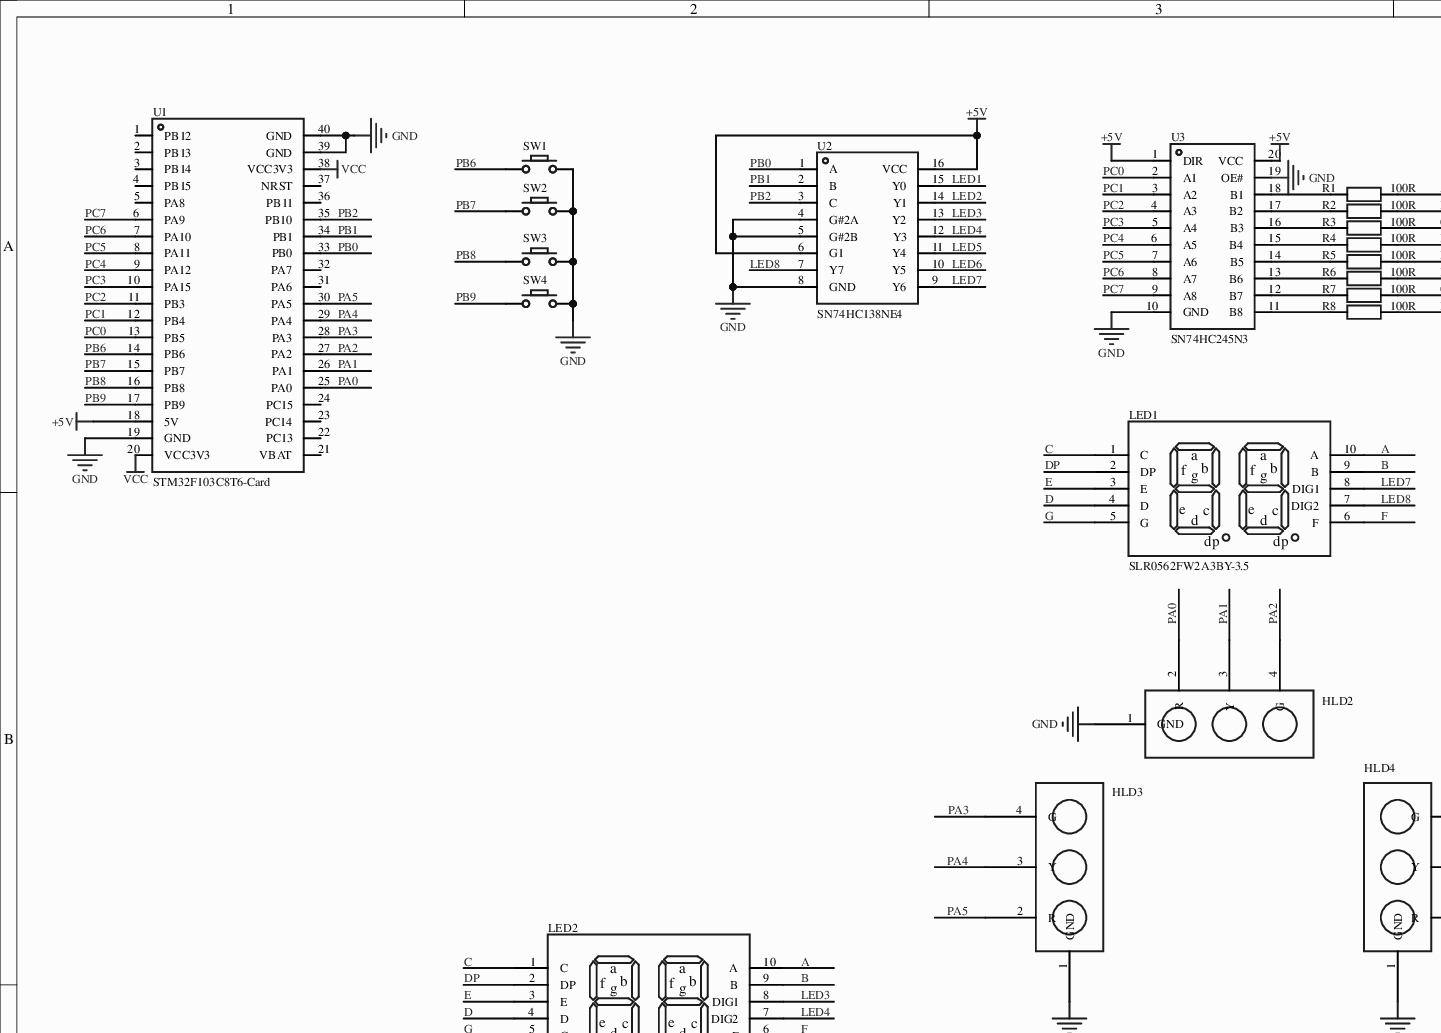
[diagram p0: MISC51569-3.schdoc, top left]
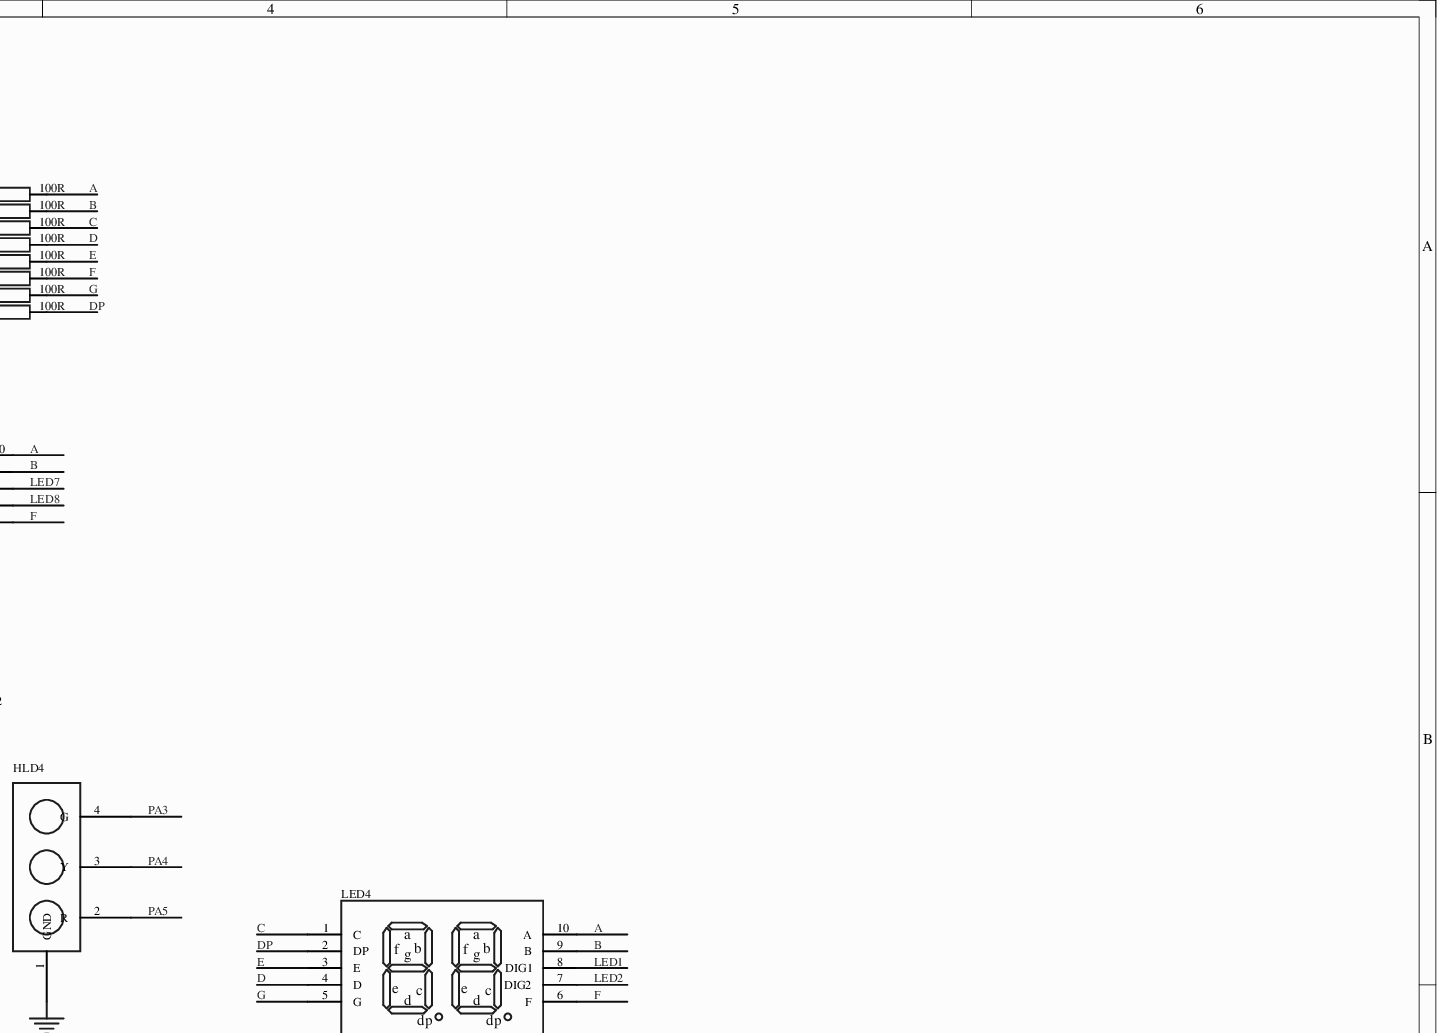
[diagram p1: MISC51569-3.schdoc, top right]
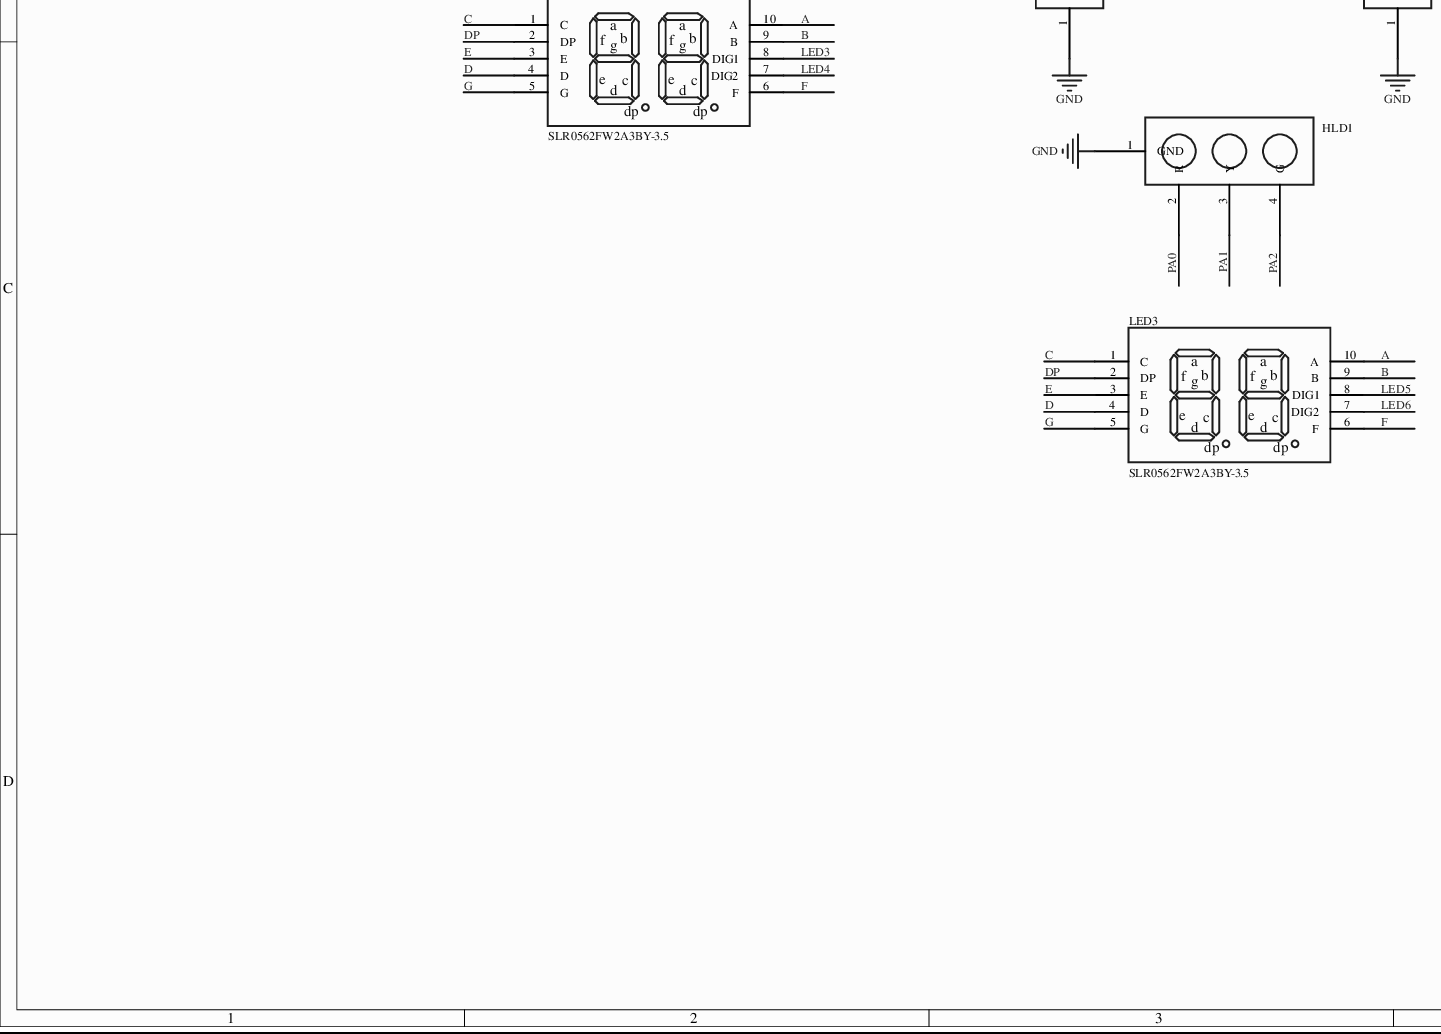
[diagram p2: MISC51569-3.schdoc, bottom left]
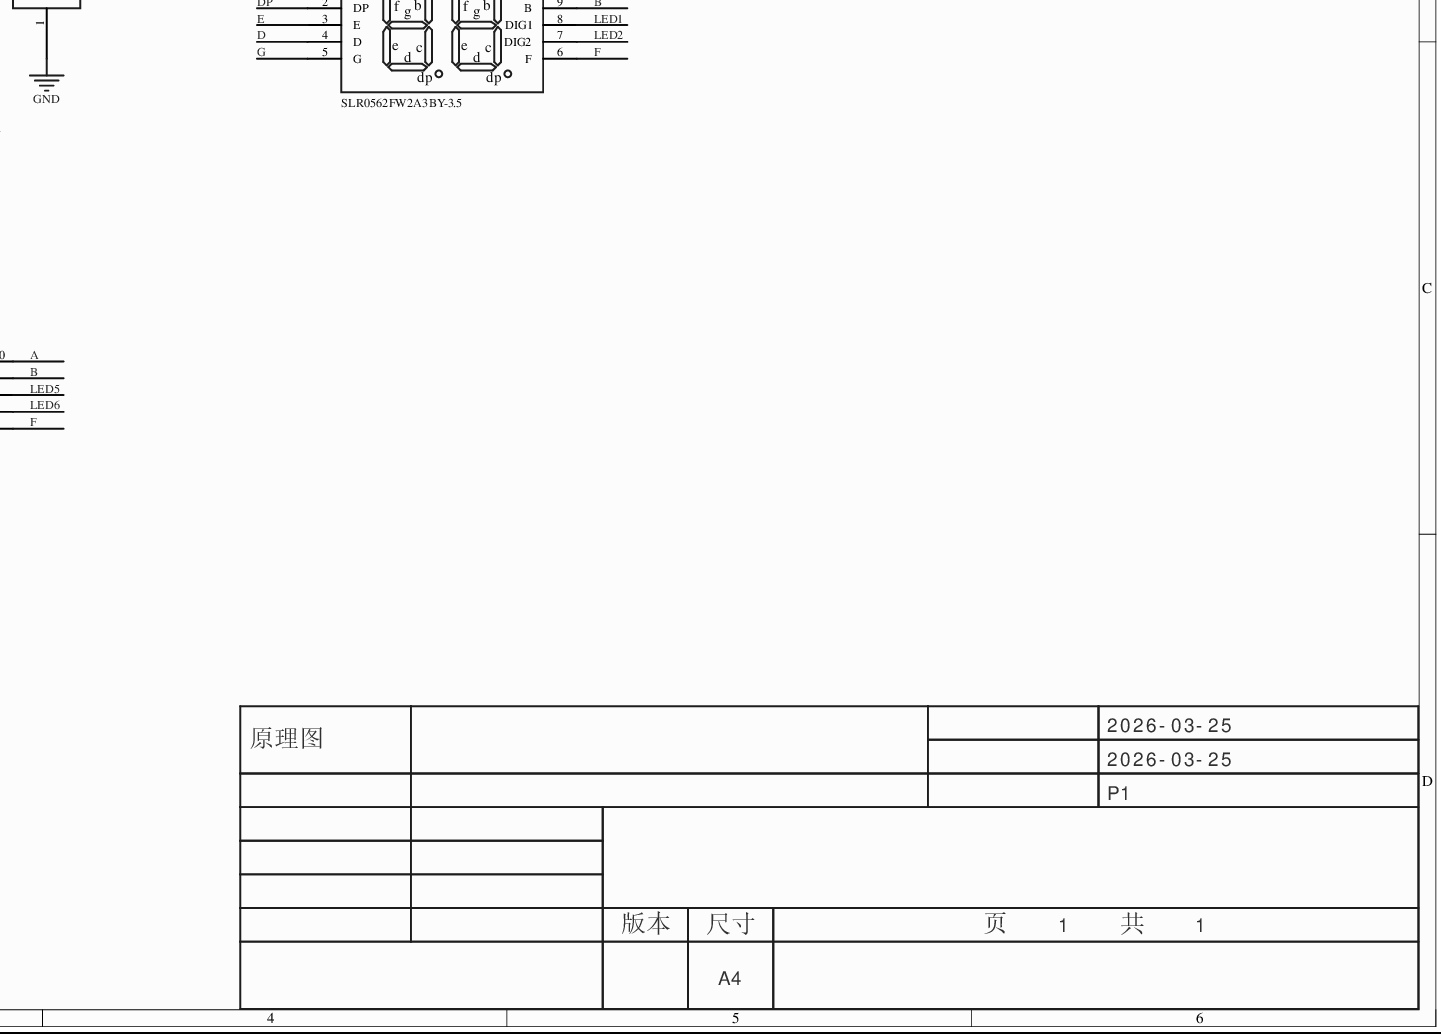
[diagram p3: MISC51569-3.schdoc, bottom right]
# Altium project MISC51569-2.PrjPcb
1 sheet, 23 parts. Net scope: global (net labels, ports and power ports of the same name join across sheets).
Board file: MISC51569.pcbdoc

## Sheet MISC51569-3.schdoc
size 420 x 297 mm; Version: V1.0; @Project Name: MISC51569; @Update Date: 2026-03-25; @Create Date: 2026-03-25; @Board Name: MISC51569; @Create Time: 20:56:41; @Page Count: 1; @Page No: 1; @Schematic Name: MISC51569; @Update Time: 20:56:41; Size: A4

### Parts
HLD1  (no value)  [SIP-04]
HLD2  (no value)  [SIP-04]
HLD3  (no value)  [SIP-04]
HLD4  (no value)  [SIP-04]
LED1  SLR0562FW2A3BY-3.5  [LED-SEG-TH_10P-L25.0-W19.0-P2.54-S15.24-BL]
LED2  SLR0562FW2A3BY-3.5  [LED-SEG-TH_10P-L25.0-W19.0-P2.54-S15.24-BL]
LED3  SLR0562FW2A3BY-3.5  [LED-SEG-TH_10P-L25.0-W19.0-P2.54-S15.24-BL]
LED4  SLR0562FW2A3BY-3.5  [LED-SEG-TH_10P-L25.0-W19.0-P2.54-S15.24-BL]
R1  100R  [Res_1/8W]
R2  100R  [Res_1/8W]
R3  100R  [Res_1/8W]
R4  100R  [Res_1/8W]
R5  100R  [Res_1/8W]
R6  100R  [Res_1/8W]
R7  100R  [Res_1/8W]
R8  100R  [Res_1/8W]
SW1  (no value)  [Key_TH_3.5x6x4.3]
SW2  (no value)  [Key_TH_3.5x6x4.3]
SW3  (no value)  [Key_TH_3.5x6x4.3]
SW4  (no value)  [Key_TH_3.5x6x4.3]
U1  STM32F103C8T6-Card  [CONN-TH_L53.3-W22.9_STM32F103C8T6-CARD]
U2  SN74HC138NE4  [PDIP-16_L19.7-W6.6-P2.54-LS7.6-BL]
U3  SN74HC245N3  [PDIP-20_L25.9-W6.6-P2.54-LS7.9-BL]

### Nets
+5V: U1.18(5V) U2.6(G1) U2.16(VCC) U3.1(DIR) U3.20(VCC)
GND: HLD1.1(GND) HLD2.1(GND) HLD3.1(GND) HLD4.1(GND) SW1.B SW2.B SW3.B SW4.B U1.19(GND) U1.39(GND) U1.40(GND) U2.4(G#2A) U2.5(G#2B) U2.8(GND) U3.10(GND) U3.19(OE#)
VCC: U1.20(VCC3V3) U1.38(VCC3V3)
A: LED1.10(A) LED2.10(A) LED3.10(A) LED4.10(A) R1.2
B: LED1.9(B) LED2.9(B) LED3.9(B) LED4.9(B) R2.2
C: LED1.1(C) LED2.1(C) LED3.1(C) LED4.1(C) R3.2
D: LED1.4(D) LED2.4(D) LED3.4(D) LED4.4(D) R4.2
DP: LED1.2(DP) LED2.2(DP) LED3.2(DP) LED4.2(DP) R8.2
E: LED1.3(E) LED2.3(E) LED3.3(E) LED4.3(E) R5.2
F: LED1.6(F) LED2.6(F) LED3.6(F) LED4.6(F) R6.2
G: LED1.5(G) LED2.5(G) LED3.5(G) LED4.5(G) R7.2
LED1: LED4.8(DIG1) U2.15(Y0)
LED2: LED4.7(DIG2) U2.14(Y1)
LED3: LED2.8(DIG1) U2.13(Y2)
LED4: LED2.7(DIG2) U2.12(Y3)
LED5: LED3.8(DIG1) U2.11(Y4)
LED6: LED3.7(DIG2) U2.10(Y5)
LED7: LED1.8(DIG1) U2.9(Y6)
LED8: LED1.7(DIG2) U2.7(Y7)
PA0: HLD1.2(R) HLD2.2(R) U1.25(PA0)
PA1: HLD1.3(Y) HLD2.3(Y) U1.26(PA1)
PA2: HLD1.4(G) HLD2.4(G) U1.27(PA2)
PA3: HLD3.4(G) HLD4.4(G) U1.28(PA3)
PA4: HLD3.3(Y) HLD4.3(Y) U1.29(PA4)
PA5: HLD3.2(R) HLD4.2(R) U1.30(PA5)
PB0: U1.33(PB0) U2.1(A)
PB1: U1.34(PB1) U2.2(B)
PB2: U1.35(PB10) U2.3(C)
PB6: SW1.A U1.14(PB6)
PB7: SW2.A U1.15(PB7)
PB8: SW3.A U1.16(PB8)
PB9: SW4.A U1.17(PB9)
PC0: U1.13(PB5) U3.2(A1)
PC1: U1.12(PB4) U3.3(A2)
PC2: U1.11(PB3) U3.4(A3)
PC3: U1.10(PA15) U3.5(A4)
PC4: U1.9(PA12) U3.6(A5)
PC5: U1.8(PA11) U3.7(A6)
PC6: U1.7(PA10) U3.8(A7)
PC7: U1.6(PA9) U3.9(A8)
NetR1_1: R1.1 U3.18(B1)
NetR2_1: R2.1 U3.17(B2)
NetR3_1: R3.1 U3.16(B3)
NetR4_1: R4.1 U3.15(B4)
NetR5_1: R5.1 U3.14(B5)
NetR6_1: R6.1 U3.13(B6)
NetR7_1: R7.1 U3.12(B7)
NetR8_1: R8.1 U3.11(B8)

Not connected (* = marked no-connect by the designer): U1 1(PB12) 2(PB13) 3(PB14) 4(PB15) 5(PA8) 21(VBAT) 22(PC13) 23(PC14) 24(PC15) 31(PA6) 32(PA7) 36(PB11) 37(NRST)

### Notes on the sheet
- 2026-03-25
- 原理图
- P1
- 版本
- 尺寸
- A4
- 页    1    共    1

### Library data of the parts
HLD1-HLD4 = RGY: AddInBom: yes; Symbol: RGY; Device: RGY; Origin Footprint: SIP-04; Design Item ID: RGY; Library Name: 红绿灯; FootprintName: SIP-04; ConvertToPcb: yes
LED1-LED4 = SLR0562FW2A3BY-3.5: 数码管位数:2位;字符尺寸(英寸):0.56;发光颜色:白色;LED极性:共阳极;; Manufacturer: SUNLIGHT(光华); AddInBom: yes; ModelId: f234e57d14da4f6ba1e64ce5b79f48750819f05c4eef4c71ace90d822a990e87; ModelName: LED-SEG-TH_0.56_2p; ModelTransform: 984.25,748.03,0,0,0,0,-3.425,3.386,-137.795; Number of Characters: 2位; Display Type: 7段; Digit/Alpha Size(inch): 0.56; Illumination Color: 白色; LED Polarity: 共阳极; Forward Voltage Drop: 3V; Symbol: SLR0562FW2A3BY-3.5; Device: SLR0562FW2A3BY-3.5; LCSC Part Name: 数码管; SupplierPart: C3036474; ManufacturerPart: SLR0562FW2A3BY-3.5; Supplier Footprint: 插件; JLCPCB Part Class: Extended Part; Datasheet: https://item.szlcsc.com/datasheet/SLR0562FW2A3BY-3.5/3587338.html; Supplier: LCSC; ConvertToPcb: yes; FootprintName: LED-SEG-TH_10P-L25.0-W19.0-P2.54-S15.24-BL; Operating Temperature: -20℃~+60℃; Length: 25mm; Width: 19mm; Height: 8mm
R1-R8 = Res_AXIAL-1/8W: Symbol: 电阻; ConvertToPcb: yes; ModelId: b2b5ae7ae4c642178fe0039925c86a3f0819f05c4eef4c71ace90d822a990e87; ModelName: RES-TH_BD1.8-L3.2-P7.20-D0.4; ModelTransform: 282.86,66.88,253.09,0,0,0,0,0,-191; Device: Res_AXIAL-1/8W; Value: 100R; AddInBom: yes; Supplier Footprint: 轴向引线; FootprintName: Res_1/8W
SW1-SW4 = Key_TH_3.5x6x4.3: ConvertToPcb: yes; ModelId: c3523f9014d949d7ba5445190a3178990819f05c4eef4c71ace90d822a990e87; ModelName: SW-TH_L6.0-W3.5-H5.0-P6.5; ModelTransform: 308.49,137.8,335.08,0,0,0,0,0,-129.92; Symbol: Key_TH_3.5x6x4.3; Device: Key_TH_3.5x6x4.3; AddInBom: yes; Supplier Footprint: 插件; FootprintName: Key_TH_3.5x6x4.3
U1 = STM32F103C8T6-Card: AddInBom: yes; Symbol: STM32F103C8T6-CARD; Device: STM32F103C8T6-Card; LCSC Part Name: STM32F103C8T6-Card; SupplierPart: C9900077949; ManufacturerPart: STM32F103C8T6-Card; Supplier Footprint: 插件; JLCPCB Part Class: Extended Part; Supplier: LCSC; ConvertToPcb: yes; FootprintName: CONN-TH_L53.3-W22.9_STM32F103C8T6-CARD
U2 = SN74HC138NE4: SN74HC138 3 线至 8 线解码器/多路信号分离器; Manufacturer: TI(德州仪器); AddInBom: yes; ModelId: 60304d8eb9b246fdb135cb3d16f241a80819f05c4eef4c71ace90d822a990e87; ModelName: PDIP-16_L19.7-W6.6-H5.1-P2.54-LS7.6-BL; ModelTransform: 787.4,311.8104,0,0,0,0,0,0,-118.11; Symbol: SN74HC138NE4; Device: SN74HC138NE4; LCSC Part Name: SN74HC138NE4; SupplierPart: C20345712; ManufacturerPart: SN74HC138NE4; Supplier Footprint: PDIP-16; JLCPCB Part Class: Extended Part; Datasheet: https://item.szlcsc.com/datasheet/SN74HC138NE4/21671239.html; Supplier: LCSC; ConvertToPcb: yes; FootprintName: PDIP-16_L19.7-W6.6-P2.54-LS7.6-BL
U3 = SN74HC245N3: 输入类型:-;工作电压:2V~6V;元件数:1;每个元件位数:8;灌电流(IOL):7.8mA;拉电流(IOH):7.8mA;; Manufacturer: TI(德州仪器); AddInBom: yes; ModelId: 8ae203acf1184a9bb7774c089354eb250819f05c4eef4c71ace90d822a990e87; ModelTransform: 1019.68308,320.8655,0,0,0,0,0,0,-118.11; output type: 三态; Voltage - Supply: 2V~6V; Number of Elements: 1; Number of Bits per Element: 8; Channel Type: 双向; Current - Output Low(IOL): 7.8mA; Logic Family: 74HC; Quiescent Current: 80uA; Propagation Delay: 21ns@4.5V,50pF; Symbol: SN74HC245N3; Device: SN74HC245N3; LCSC Part Name: SN74HC245N3; SupplierPart: C3587488; ManufacturerPart: SN74HC245N3; Supplier Footprint: PDIP-20; JLCPCB Part Class: Extended Part; Datasheet: https://item.szlcsc.com/datasheet/SN74HC245N3/4154202.html; Supplier: LCSC; ConvertToPcb: yes; FootprintName: PDIP-20_L25.9-W6.6-P2.54-LS7.9-BL; ModelName: PDIP-20_L25.9-W6.6-P2.54-LS7.9-BL; Input type: -; Current - Output High(IOH): 7.8mA; Operating Temperature: -40℃~+85℃